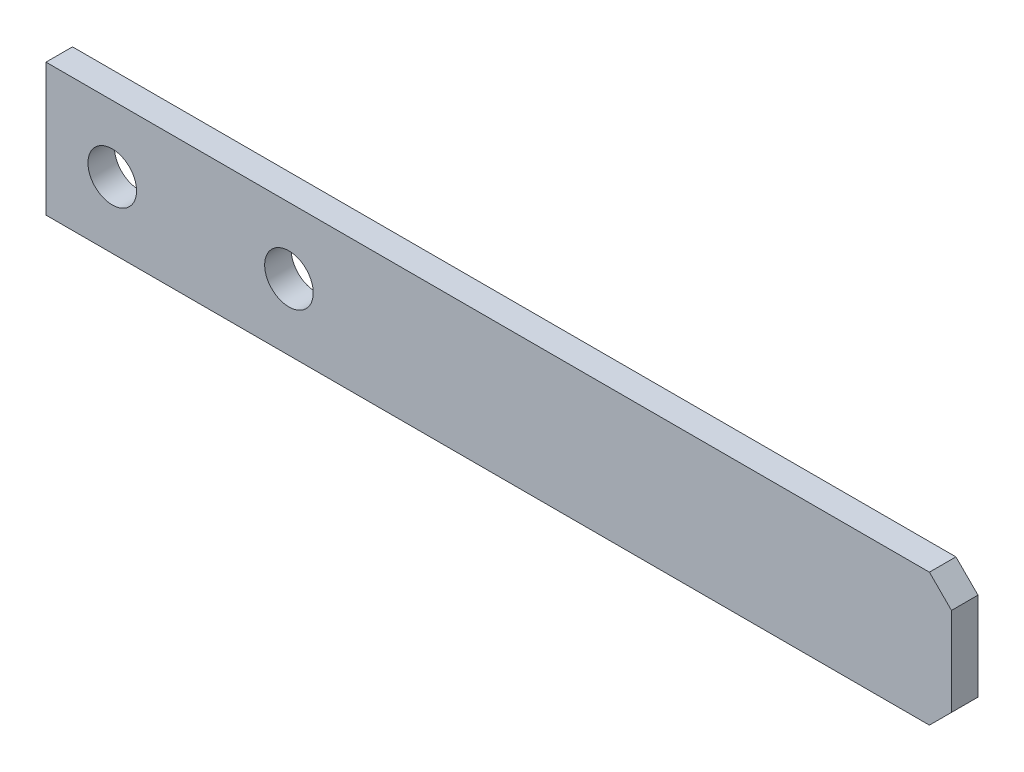
from build123d import *

# Parameters (mm, degrees)
SKETCH1_R           = 5.5
BOSS_EXTRUDE1_DEPTH = 6


with BuildPart() as part:
    # Sketch1 → Boss-Extrude1 (new body)
    with BuildSketch(Plane.XY.offset(3)):
        Polygon((102.5, -10), (102.5, 10), (97.5, 15), (-102.5, 15), (-102.5, -15), (97.5, -15), align=None)
        with Locations(Location((-87.5, 0, 0), (0, 0, 180))):
            Circle(SKETCH1_R, mode=Mode.SUBTRACT)
        with Locations(Location((-47.5, 0, 0), (0, 0, 180))):
            Circle(SKETCH1_R, mode=Mode.SUBTRACT)
    extrude(amount=-BOSS_EXTRUDE1_DEPTH)


solid = part.part
